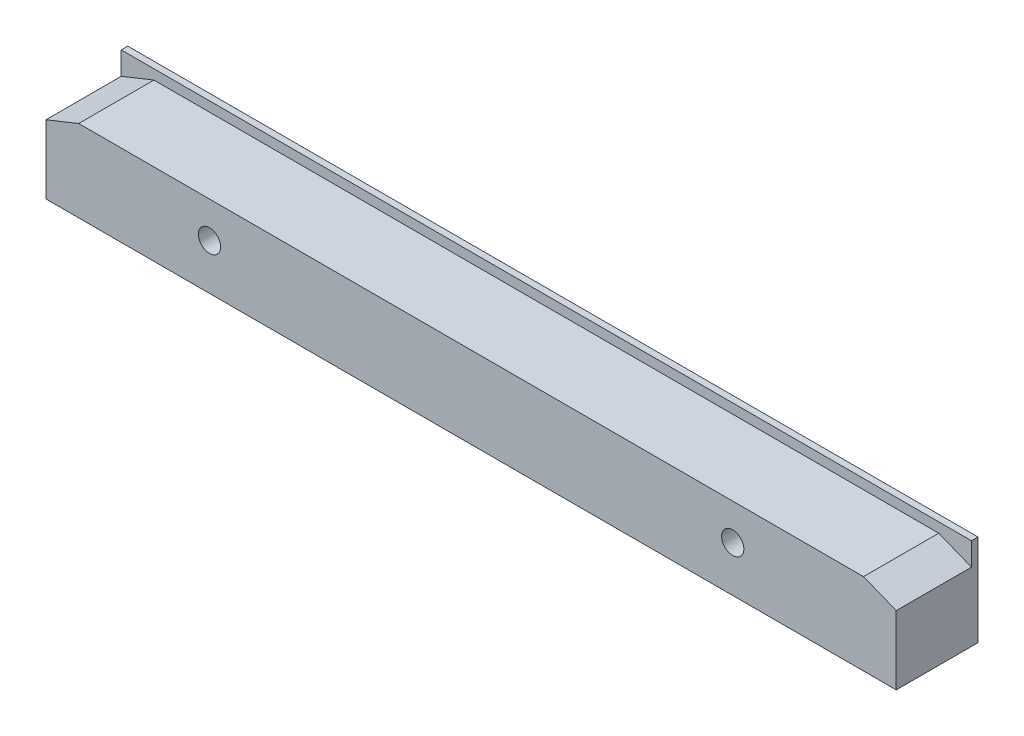
SolidWorks part; units mm, degrees
ref_plane "前视基准面" through (0, 0, 0) normal (0, 0, 1) x (1, 0, 0)
ref_plane "上视基准面" through (0, 0, 0) normal (0, 1, 0) x (1, 0, 0)
ref_plane "右视基准面" through (0, 0, 0) normal (1, 0, 0) x (0, 0, -1)
sketch "草图1" plane through (0, 0, 0) normal (0, 0, 1) x (1, 0, 0)
  line L1 (-65, 7) -> (65, 7)
  line L2 (-65, 7) -> (-65, -7)
  line L3 (-65, -7) -> (65, -7)
  line L4 (65, 7) -> (65, -7)
  line L5 (-65, 7) -> (65, -7) construction
  line L6 (-65, -7) -> (65, 7) construction
  point P0 (0, 0)
  dimension "D1" = 130
  dimension "D2" = 14
extrude "凸台-拉伸1" add sketch "草图1" along normal blind 12.5
sketch "草图2" plane through (65, 0, 0) normal (1, 0, 0) x (0, 0, -1)
  line L0 (0, -7) -> (0, 7) construction
  line L1 (-12.5, 7) -> (-1, 7)
  line L2 (-12.5, 7) -> (-12.5, 5.5)
  line L3 (-12.5, 5.5) -> (-1, 5.5)
  line L4 (-1, 7) -> (-1, 5.5)
  dimension "D1" = 1
  dimension "D2" = 1.5
extrude "切除-拉伸1" cut sketch "草图2" against normal through all
chamfer "倒角3" distance 2 distance2 5 1 edges at (65, 5.5, 6.75)
chamfer "倒角4" distance 5 distance2 2 1 edges at (-65, 5.5, 6.75)
hole_wizard "打孔尺寸根据内六角圆柱头螺钉的类型1" positions "草图4" profile "草图3" counterbore size "M3" standard "Gb" end condition through all
sketch "草图4" plane through (0, 0, 0) normal (0, 0, -1) x (-1, 0, 0)
  line L0 (-65, -7) -> (-65, 7) construction
  line L1 (65, 7) -> (65, -7) construction
  point P0 (-40, 0)
  point P2 (40, 0)
  dimension "D1" = 25
  dimension "D2" = 25
sketch "草图3" plane through (40, 0, 0) normal (1, 0, 0) x (0, 1, 0)
  line L0 (0, 0) -> (0, 12.5)
  line L1 (0, 12.5) -> (1.7, 12.5)
  line L3 (1.7, 12.5) -> (1.7, 3.4)
  line L4 (1.7, 3.4) -> (3, 3.4)
  line L5 (3, 3.4) -> (3, 0)
  line L7 (3, 0) -> (0, 0)
  line L11 (0, -6.35) -> (0, 107.95) construction
  dimension "通孔孔直径" = 3.4
  dimension "通孔孔深度" = 12.5
  dimension "柱形沉头孔直径" = 6
  dimension "柱形沉头孔深度" = 3.4
